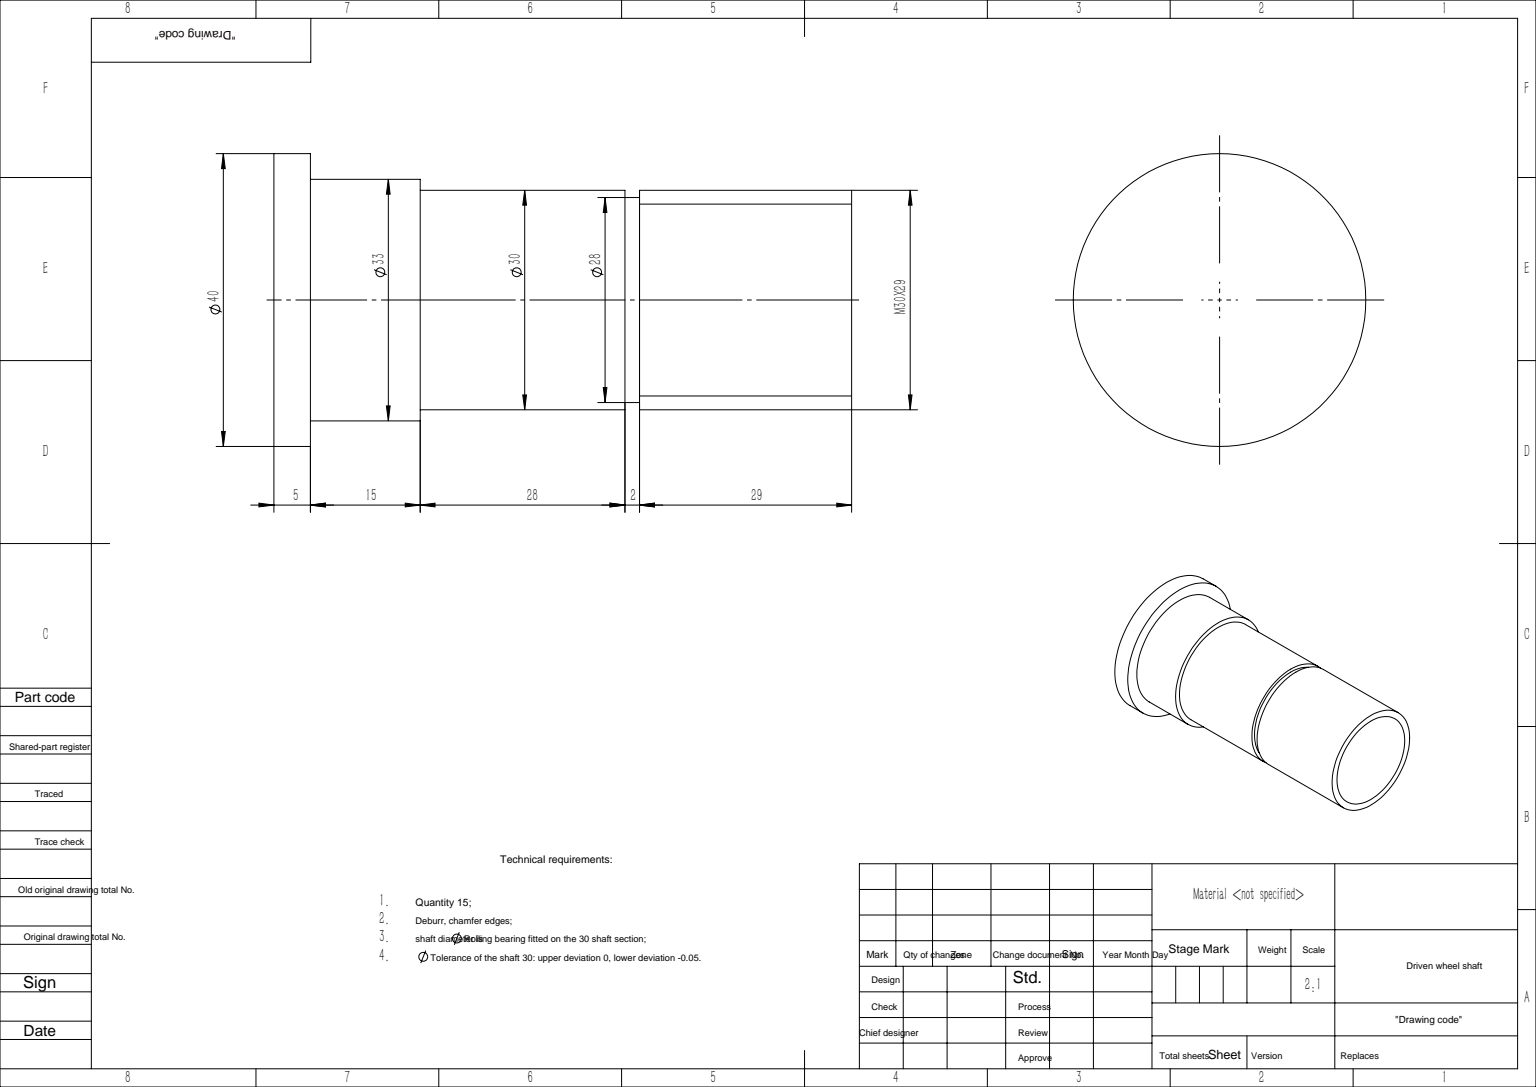
SolidWorks part; units mm, degrees
ref_plane "前视基准面" through (0, 0, 0) normal (0, 0, 1) x (1, 0, 0)
ref_plane "上视基准面" through (0, 0, 0) normal (0, 1, 0) x (1, 0, 0)
ref_plane "右视基准面" through (0, 0, 0) normal (1, 0, 0) x (0, 0, -1)
sketch "草图1" plane through (0, 0, 0) normal (0, 0, 1) x (1, 0, 0)
  line L1 (0, 0) -> (0, 20)
  line L2 (0, 20) -> (5, 20)
  line L3 (5, 20) -> (5, 16.5)
  line L4 (5, 16.5) -> (20, 16.5)
  line L5 (20, 16.5) -> (20, 15)
  line L6 (79, 0) -> (0, 0)
  line L7 (20, 15) -> (79, 15)
  line L8 (79, 15) -> (79, 0)
  dimension "D1" = 20
  dimension "D2" = 16.5
  dimension "D3" = 5
  dimension "D4" = 15
  dimension "D5" = 15
  dimension "D6" = 59
revolve "旋转1" add sketch "草图1" angle 360 about L6
cosmetic thread "装饰螺纹线1" parameters "D1"=29, "D2"=26.211
sketch "草图3" plane through (79, 0, 0) normal (1, 0, 0) x (0, 0, -1)
  circle A0 centre (0, 0) radius 15 construction
  circle A1 centre (0, 0) radius 15
  circle A2 centre (0, 0) radius 14
  dimension "D1" = 1
extrude "切除-拉伸1" cut sketch "草图3" along normal blind 2 from offset 31
